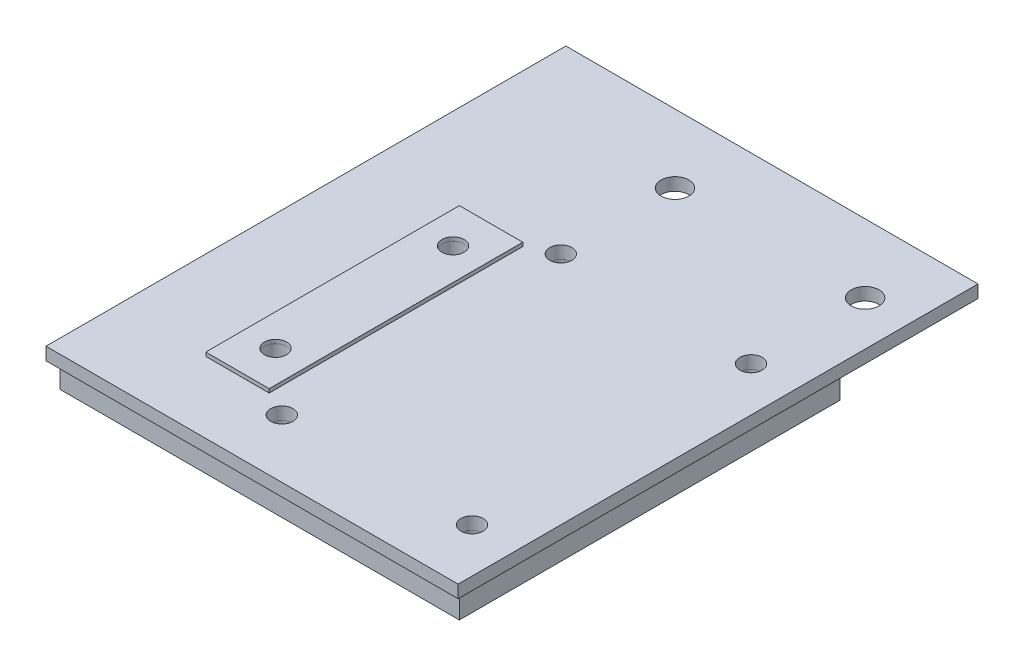
SolidWorks part; units mm, degrees
material "A3"
ref_plane "前视基准面" through (0, 0, 0) normal (0, 0, 1) x (1, 0, 0)
ref_plane "上视基准面" through (0, 0, 0) normal (0, 1, 0) x (1, 0, 0)
ref_plane "右视基准面" through (0, 0, 0) normal (1, 0, 0) x (0, 0, -1)
sketch "草图1" plane through (0, 0, 0) normal (0, 1, 0) x (1, 0, 0)
  line L1 (-157.5, -150) -> (157.5, -150)
  line L2 (-157.5, -150) -> (-157.5, 150)
  line L3 (-157.5, 150) -> (157.5, 150)
  line L4 (157.5, -150) -> (157.5, 150)
  line L5 (-157.5, -150) -> (157.5, 150) construction
  line L6 (-157.5, 150) -> (157.5, -150) construction
  point P0 (0, 0)
  dimension "D1" = 300
  dimension "D2" = 315
extrude "凸台-拉伸1" add sketch "草图1" along normal blind 20
sketch "草图2" plane through (0, 20, 0) normal (0, 1, 0) x (1, 0, 0)
  line L1 (162.5, -156) -> (-162.5, -156)
  line L2 (162.5, -156) -> (162.5, 254)
  line L3 (162.5, 254) -> (-162.5, 254)
  line L4 (-162.5, -156) -> (-162.5, 254)
  line L5 (162.5, -156) -> (-162.5, 254) construction
  line L6 (162.5, 254) -> (-162.5, -156) construction
  line L7 (-157.5, -150) -> (157.5, -150) construction
  point P0 (0, 49)
  dimension "D1" = 410
  dimension "D2" = 325
  dimension "D3" = 6
extrude "凸台-拉伸2" add sketch "草图2" along normal blind 10 separate body
sketch "草图3" plane through (0, 30, 0) normal (0, 1, 0) x (1, 0, 0)
  line L0 (162.5, -156) -> (162.5, 254) construction
  line L1 (-92.5, -100) -> (-42.5, -100)
  line L2 (-92.5, -100) -> (-92.5, 100)
  line L3 (-92.5, 100) -> (-42.5, 100)
  line L4 (-42.5, -100) -> (-42.5, 100)
  line L5 (-92.5, -100) -> (-42.5, 100) construction
  line L6 (-92.5, 100) -> (-42.5, -100) construction
  point P0 (-67.5, 0)
  dimension "D1" = 200
  dimension "D2" = 50
  dimension "D3" = 230
extrude "凸台-拉伸3" add sketch "草图3" along normal blind 3 separate body
sketch "草图4" plane through (0, 0, 0) normal (0, -1, 0) x (1, 0, 0)
  line L0 (157.5, 150) -> (157.5, -150) construction
  line L1 (-142.5, -50) -> (-112.5, -50)
  line L2 (-142.5, -50) -> (-142.5, 50)
  line L3 (-142.5, 50) -> (-112.5, 50)
  line L4 (-112.5, -50) -> (-112.5, 50)
  line L5 (-142.5, -50) -> (-112.5, 50) construction
  line L6 (-142.5, 50) -> (-112.5, -50) construction
  point P0 (-127.5, 0)
  dimension "D1" = 100
  dimension "D2" = 30
  dimension "D3" = 270
extrude "凸台-拉伸4" add sketch "草图4" along normal blind 30 separate body
hole_wizard "M20 螺纹孔1" positions "草图6" profile "草图7" tap size "M20" standard "GB"
sketch "草图6" plane through (0, 33, 0) normal (0, 1, 0) x (1, 0, 0)
  line L0 (52.5, 254) -> (52.5, 0) construction
  line L1 (162.5, 254) -> (-162.5, 254) construction
  line L2 (52.5, 0) -> (0, 0) construction
  line L4 (162.5, -156) -> (162.5, 254) construction
  point P0 (-67.5, 70)
  point P2 (-22.5, 110)
  point P15 (-22.5, -110)
  point P16 (-67.5, -70)
  point P17 (127.5, -110)
  point P18 (127.5, 110)
  dimension "D1" = 110
  dimension "D2" = 150
  dimension "D3" = 220
  dimension "D4" = 140
  dimension "D5" = 120
sketch "草图7" plane through (-67.5, 33, -70) normal (1, 0, 0) x (0, 0, 1)
  line L0 (0, 0) -> (0, 57.7575)
  line L1 (0, 57.7575) -> (8.75, 52.5)
  line L2 (8.75, 52.5) -> (8.75, 0)
  line L5 (8.75, 0) -> (0, 0)
  line L10 (0, 57.7575) -> (-8.75, 52.5) construction
  line L11 (0, -6.35) -> (0, 107.95) construction
  dimension "螺纹孔钻头直径" = 17.5
  dimension "螺纹孔钻头深度" = 52.5
  dimension "导头角度" = 118
cosmetic thread "孔螺蚊线1" parameters "D1"=40, "D2"=20
cosmetic thread "孔螺蚊线2" parameters "D1"=40, "D2"=20
cosmetic thread "孔螺蚊线3" parameters "D1"=40, "D2"=20
cosmetic thread "孔螺蚊线4" parameters "D1"=40, "D2"=20
cosmetic thread "孔螺蚊线5" parameters "D1"=40, "D2"=20
cosmetic thread "孔螺蚊线6" parameters "D1"=40, "D2"=20
sketch "草图5" plane through (0, 30, 0) normal (0, 1, 0) x (1, 0, 0)
  line L0 (52.5, -156) -> (52.5, 254) construction
  line L1 (-162.5, -156) -> (162.5, -156) construction
  line L2 (162.5, 254) -> (-162.5, 254) construction
  line L3 (162.5, -156) -> (162.5, 254) construction
  circle A0 centre (-22.5, 200) radius 11
  circle A1 centre (127.5, 200) radius 11
  circle A2 centre (127.5, 110) radius 8.75 construction
  dimension "D1" = 22
  dimension "D3" = 75
  dimension "D4" = 90
  dimension "D2" = 110
extrude "切除-拉伸1" cut sketch "草图5" against normal through all
ref_plane "基准面1" through (0, 0, 0) normal (0, 0, 1) x (1, 0, 0)
